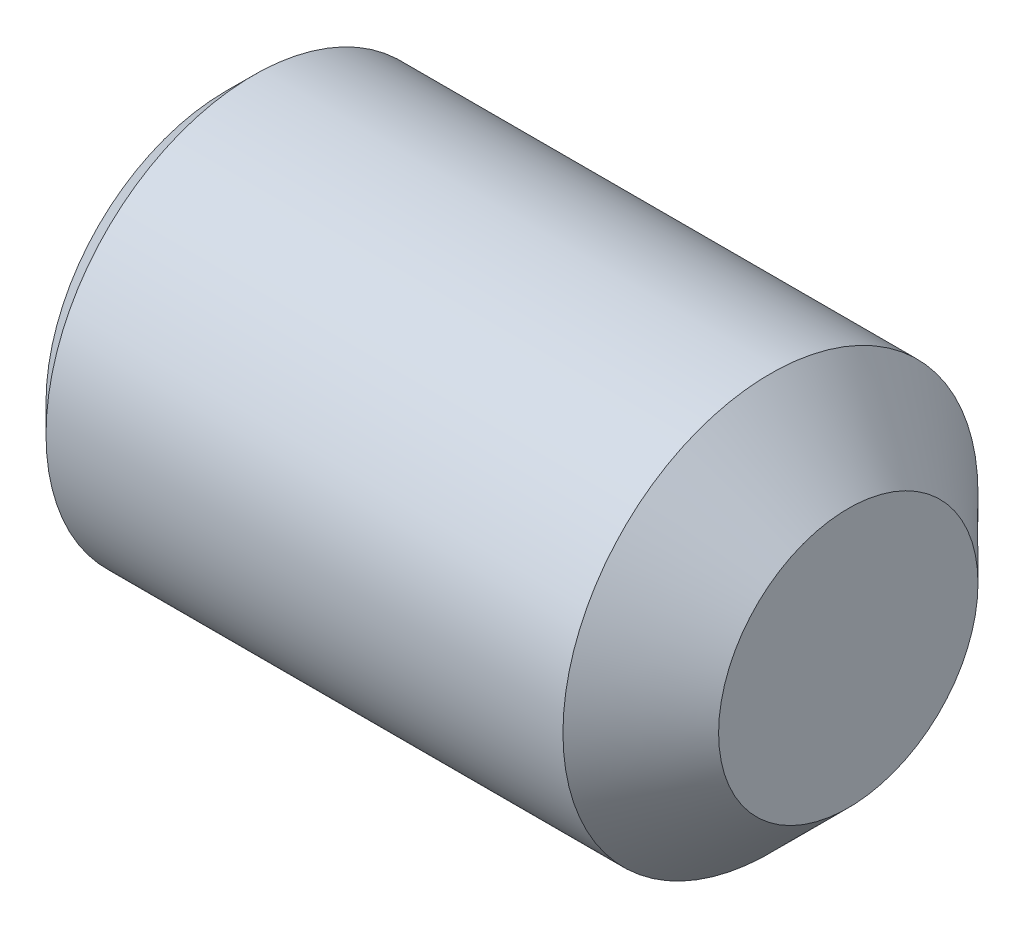
from build123d import *

# Parameters (mm, degrees)
CUT_EXTRUDE1_DEPTH = 1.5


with BuildPart() as part:
    # Sketch1 → Boss-Revolve (revolve)
    with BuildSketch(Plane.XY, mode=Mode.PRIVATE) as boss_revolve_sk:
        Polygon((0, 0), (6, 0), (6, 1.25), (5.25, 2), (0.268, 2), (0, 1.732), align=None)
    revolve(boss_revolve_sk.sketch.rotate(Axis((-0.277777778, 0, 0), (1, 0, 0)), 90), axis=Axis((-0.277777778, 0, 0), (1, 0, 0)))

    # Sketch2 → Cut-Extrude1 (cut)
    with BuildSketch(Plane.ZY):
        Polygon((-0.575, -0.995929214), (0.575, -0.995929214), (1.15, 0), (0.575, 0.995929214), (-0.575, 0.995929214), (-1.15, 0), align=None)
    extrude(amount=-CUT_EXTRUDE1_DEPTH, mode=Mode.SUBTRACT)

    # Sketch4 → Cut-Revolve2 (revolve, cut)
    with BuildSketch(Plane.XY, mode=Mode.PRIVATE) as cut_revolve2_sk:
        Polygon((1.5, 0.995929214), (2.075, 0), (1.5, 0), align=None)
    revolve(cut_revolve2_sk.sketch.rotate(Axis((-0.277777778, 0, 0), (1, 0, 0)), 90), axis=Axis((-0.277777778, 0, 0), (1, 0, 0)), mode=Mode.SUBTRACT)


solid = part.part
